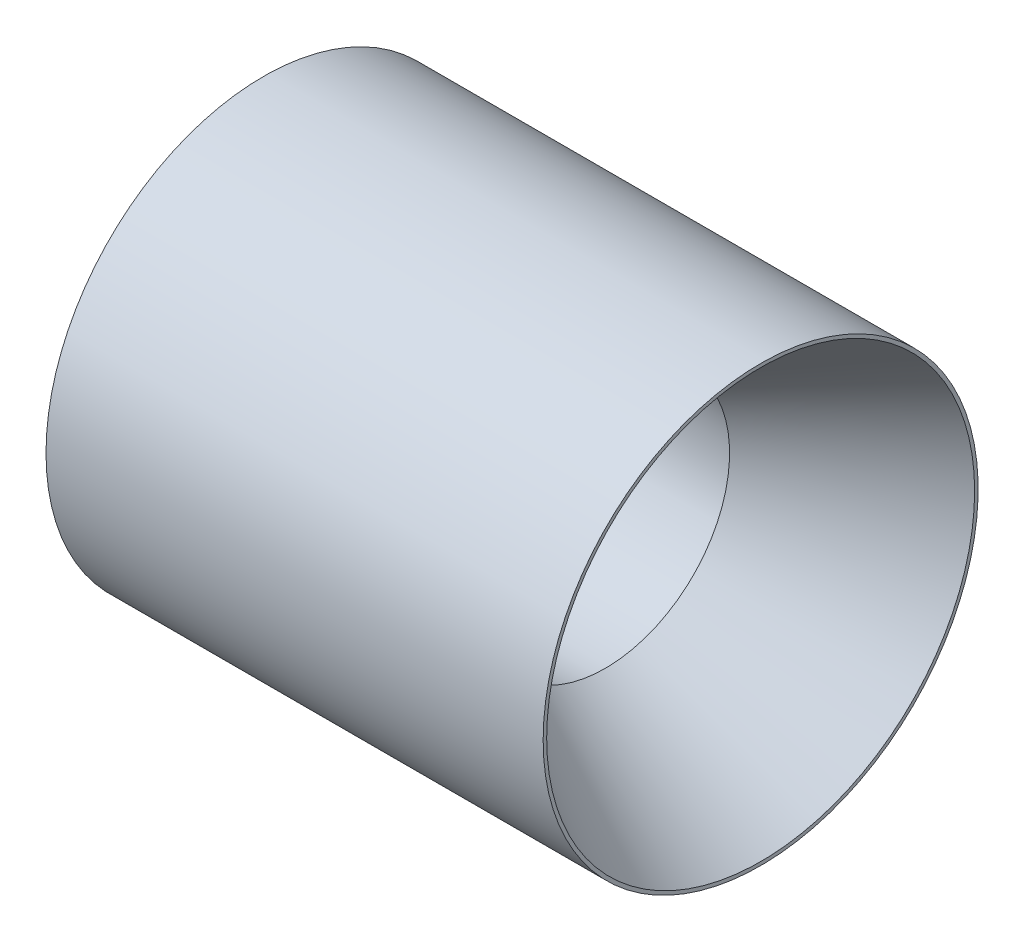
SolidWorks part; units mm, degrees
material "S45C"
ref_plane "Front Plane" through (0, 0, 0) normal (0, 0, 1) x (1, 0, 0)
ref_plane "Top Plane" through (0, 0, 0) normal (0, 1, 0) x (1, 0, 0)
ref_plane "Right Plane" through (0, 0, 0) normal (1, 0, 0) x (0, 0, -1)
sketch "Sketch1" plane through (0, 0, 0) normal (0, 0, 1) x (1, 0, 0)
  line L0 (0, 0) -> (80.6164, 0) construction
  line L1 (0, 4) -> (11, 4)
  line L2 (11, 4) -> (16, 6.8868)
  line L3 (16, 6.8868) -> (16, 7)
  line L4 (16, 7) -> (0, 7)
  line L5 (0, 7) -> (0, 4)
  dimension "D1" = 7
  dimension "D2" = 4
  dimension "D3" = 16
  dimension "D4" = 11
  dimension "D5" = 30
revolve "Revolve1" add sketch "Sketch1" angle 360 about L0
